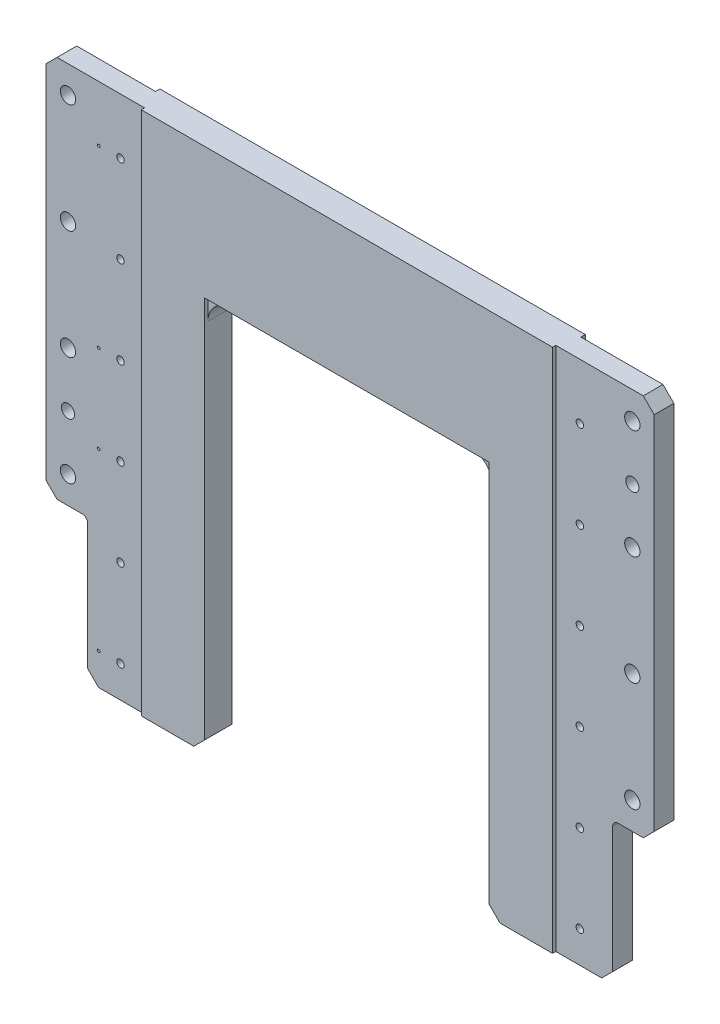
from build123d import *

# Parameters (mm, degrees)
BOSS_EXTRUDE1_DEPTH             = 22
SKETCH2_W                       = 85
SKETCH2_H                       = 480
SKETCH2_W_2                     = 82
CUT_EXTRUDE1_DEPTH              = 4
M8_TAPPED_HOLE1_AT_2_COUNT      = 2
M8_TAPPED_HOLE1_AT_2_PITCH      = 80
M8_TAPPED_HOLE1_AT_3_COUNT      = 2
M8_TAPPED_HOLE1_AT_3_PITCH      = 160
M8_TAPPED_HOLE1_AT_4_COUNT      = 2
M8_TAPPED_HOLE1_AT_4_PITCH      = 240
M8_TAPPED_HOLE1_AT_5_COUNT      = 2
M8_TAPPED_HOLE1_AT_5_PITCH      = 320
M8_TAPPED_HOLE1_AT_6_COUNT      = 2
M8_TAPPED_HOLE1_AT_6_PITCH      = 80
F_14_0_14_DIAMETER_HOLE1_D      = 14
F_7_0_7_DIAMETER_HOLE1_D        = 7
F_7_0_7_DIAMETER_HOLE1_DEPTH    = 4
M3_TAPPED_HOLE1_D               = 2.5
M3_TAPPED_HOLE1_DEPTH           = 18
M3_TAPPED_HOLE1_ON_FACE_2_D     = 2.5
M3_TAPPED_HOLE1_ON_FACE_2_DEPTH = 18
F_12_0_12_DIAMETER_HOLE1_D      = 12
CUT_EXTRUDE2_REACH              = 736.752
SKETCH9_W                       = 38
SKETCH9_H                       = 130
CUT_EXTRUDE2_DIRECTION_2_DEPTH  = 5
FILLET1_R                       = 5
CHAMFER1_SIZE                   = 10
BOSS_EXTRUDE2_DEPTH             = 3


with BuildPart() as part:
    # Sketch1 → Boss-Extrude1 (new body)
    with BuildSketch(Plane.XY):
        with BuildLine():
            Line((0, 10), (0, 470))
            Line((0, 470), (10, 480))
            Line((10, 480), (546, 480))
            Line((546, 480), (556, 470))
            Line((556, 470), (556, 10))
            Line((556, 10), (546, 0))
            Line((546, 0), (418, 0))
            Line((418, 0), (408, 10))
            Line((408, 10), (408, 340))
            ThreePointArc((408, 340), (402.142135624, 354.142135624), (388, 360))
            Line((388, 360), (168, 360))
            ThreePointArc((168, 360), (153.857864376, 354.142135624), (148, 340))
            Line((148, 340), (148, 10))
            Line((148, 10), (138, 0))
            Line((138, 0), (10, 0))
            Line((10, 0), (0, 10))
        make_face()
    extrude(amount=BOSS_EXTRUDE1_DEPTH)

    # Sketch2 → Cut-Extrude1 (cut)
    with BuildSketch(Plane(origin=(0, 0, 0), x_dir=(-1, 0, 0), z_dir=(0, 0, -1))):
        with Locations((-513.5, 240)):
            Rectangle(SKETCH2_W, SKETCH2_H)
        with Locations((-41, 240)):
            Rectangle(SKETCH2_W_2, SKETCH2_H)
    extrude(amount=-CUT_EXTRUDE1_DEPTH, mode=Mode.SUBTRACT)

    # Sketch3 → M8 Tapped Hole1 (revolve, cut)
    with BuildSketch(Plane(origin=(488, 349, 4), x_dir=(0, 1, 0), z_dir=(1, 0, 0))):
        Polygon((0, 0), (0, 21.712990915), (3.4, 19.75), (3.4, 0), align=None)
    m8_tapped_hole1 = revolve(axis=Axis((488, 349, -2.35), (0, 0, 1)), mode=Mode.SUBTRACT)

    # M8 Tapped Hole1 at 2: M8 Tapped Hole1 ×2
    with Locations(*[(0, -i * M8_TAPPED_HOLE1_AT_2_PITCH, 0) for i in range(1, M8_TAPPED_HOLE1_AT_2_COUNT)]):
        add(m8_tapped_hole1, mode=Mode.SUBTRACT)

    # M8 Tapped Hole1 at 3: M8 Tapped Hole1 ×2
    with Locations(*[(0, -i * M8_TAPPED_HOLE1_AT_3_PITCH, 0) for i in range(1, M8_TAPPED_HOLE1_AT_3_COUNT)]):
        add(m8_tapped_hole1, mode=Mode.SUBTRACT)

    # M8 Tapped Hole1 at 4: M8 Tapped Hole1 ×2
    with Locations(*[(0, -i * M8_TAPPED_HOLE1_AT_4_PITCH, 0) for i in range(1, M8_TAPPED_HOLE1_AT_4_COUNT)]):
        add(m8_tapped_hole1, mode=Mode.SUBTRACT)

    # M8 Tapped Hole1 at 5: M8 Tapped Hole1 ×2
    with Locations(*[(0, -i * M8_TAPPED_HOLE1_AT_5_PITCH, 0) for i in range(1, M8_TAPPED_HOLE1_AT_5_COUNT)]):
        add(m8_tapped_hole1, mode=Mode.SUBTRACT)

    # M8 Tapped Hole1 at 6: M8 Tapped Hole1 ×2
    with Locations(*[(0, i * M8_TAPPED_HOLE1_AT_6_PITCH, 0) for i in range(1, M8_TAPPED_HOLE1_AT_6_COUNT)]):
        add(m8_tapped_hole1, mode=Mode.SUBTRACT)

    # Mirror1: M8 Tapped Hole1 across plane
    add(m8_tapped_hole1.mirror(Plane(origin=(278, 0, 0), x_dir=(0, 0, 1), z_dir=(1, 0, 0))), mode=Mode.SUBTRACT)

    # Mirror1 copy 1 sketch → Mirror1 copy 1 (revolve, cut)
    with BuildSketch(Plane(origin=(68, 269, 4), x_dir=(0, 1, 0), z_dir=(-1, 0, 0))):
        Polygon((0, 0), (0, -21.712990915), (3.4, -19.75), (3.4, 0), align=None)
    revolve(axis=Axis((68, 269, -2.35), (0, 0, -1)), mode=Mode.SUBTRACT)

    # Mirror1 copy 2 sketch → Mirror1 copy 2 (revolve, cut)
    with BuildSketch(Plane(origin=(68, 189, 4), x_dir=(0, 1, 0), z_dir=(-1, 0, 0))):
        Polygon((0, 0), (0, -21.712990915), (3.4, -19.75), (3.4, 0), align=None)
    revolve(axis=Axis((68, 189, -2.35), (0, 0, -1)), mode=Mode.SUBTRACT)

    # Mirror1 copy 3 sketch → Mirror1 copy 3 (revolve, cut)
    with BuildSketch(Plane(origin=(68, 109, 4), x_dir=(0, 1, 0), z_dir=(-1, 0, 0))):
        Polygon((0, 0), (0, -21.712990915), (3.4, -19.75), (3.4, 0), align=None)
    revolve(axis=Axis((68, 109, -2.35), (0, 0, -1)), mode=Mode.SUBTRACT)

    # Mirror1 copy 4 sketch → Mirror1 copy 4 (revolve, cut)
    with BuildSketch(Plane(origin=(68, 29, 4), x_dir=(0, 1, 0), z_dir=(-1, 0, 0))):
        Polygon((0, 0), (0, -21.712990915), (3.4, -19.75), (3.4, 0), align=None)
    revolve(axis=Axis((68, 29, -2.35), (0, 0, -1)), mode=Mode.SUBTRACT)

    # Mirror1 copy 5 sketch → Mirror1 copy 5 (revolve, cut)
    with BuildSketch(Plane(origin=(68, 429, 4), x_dir=(0, 1, 0), z_dir=(-1, 0, 0))):
        Polygon((0, 0), (0, -21.712990915), (3.4, -19.75), (3.4, 0), align=None)
    revolve(axis=Axis((68, 429, -2.35), (0, 0, -1)), mode=Mode.SUBTRACT)

    # Ø14.0 (14) Diameter Hole1 (through all)
    with Locations(Plane(origin=(536, 455, 4), x_dir=(-1, 0, 0), z_dir=(0, 0, -1))):
        with Locations((0, 0), (0, -100), (0, -200), (0, -300)):
            f_14_0_14_diameter_hole1 = Hole(F_14_0_14_DIAMETER_HOLE1_D / 2)

    # Mirror2: Ø14.0 (14) Diameter Hole1 across plane
    add(f_14_0_14_diameter_hole1.mirror(Plane.ZY.offset(-278)), mode=Mode.SUBTRACT)

    # Ø7.0 (7) Diameter Hole1
    with Locations(Plane(origin=(48, 429, 4), x_dir=(-1, 0, 0), z_dir=(0, 0, -1))):
        with Locations((0, 0), (0, -160), (0, -240), (0, -400)):
            Hole(F_7_0_7_DIAMETER_HOLE1_D / 2, depth=F_7_0_7_DIAMETER_HOLE1_DEPTH)

    # M3 Tapped Hole1
    with Locations(Plane(origin=(48, 429, 4), x_dir=(-1, 0, 0), z_dir=(0, 0, -1))):
        with Locations((0, 0), (0, -240)):
            Hole(M3_TAPPED_HOLE1_D / 2, depth=M3_TAPPED_HOLE1_DEPTH)

    # M3 Tapped Hole1 on face 2
    with Locations(Plane(origin=(48, 269, 8), x_dir=(-1, 0, 0), z_dir=(0, 0, -1))):
        with Locations((0, 0), (0, -240)):
            Hole(M3_TAPPED_HOLE1_ON_FACE_2_D / 2, depth=M3_TAPPED_HOLE1_ON_FACE_2_DEPTH)

    # Ø12.0 (12) Diameter Hole1 (through all)
    with Locations(Plane(origin=(20, 205, 4), x_dir=(-1, 0, 0), z_dir=(0, 0, -1))):
        with Locations((0, 0), (-516, 200)):
            Hole(F_12_0_12_DIAMETER_HOLE1_D / 2)

    # Sketch9 → Cut-Extrude2 (cut, up to next)
    with BuildSketch(Plane(origin=(0, 0, 4), x_dir=(-1, 0, 0), z_dir=(0, 0, -1)), mode=Mode.PRIVATE) as cut_extrude2_sk1:
        with Locations((-537, 65)):
            Rectangle(SKETCH9_W, SKETCH9_H)
    cut_extrude2_tool1 = extrude(cut_extrude2_sk1.sketch, amount=-CUT_EXTRUDE2_REACH, mode=Mode.PRIVATE) & part.part
    # Sketch9 → Cut-Extrude2 (cut, up to next)
    with BuildSketch(Plane(origin=(0, 0, 4), x_dir=(-1, 0, 0), z_dir=(0, 0, -1)), mode=Mode.PRIVATE) as cut_extrude2_sk2:
        with Locations((-19, 65)):
            Rectangle(SKETCH9_W, SKETCH9_H)
    cut_extrude2_tool2 = extrude(cut_extrude2_sk2.sketch, amount=-CUT_EXTRUDE2_REACH, mode=Mode.PRIVATE) & part.part
    add(cut_extrude2_tool1.solids().sort_by_distance((537, 65, 4))[0], mode=Mode.SUBTRACT)
    add(cut_extrude2_tool2.solids().sort_by_distance((19, 65, 4))[0], mode=Mode.SUBTRACT)

    # Sketch9 → Cut-Extrude2 direction 2 (cut)
    with BuildSketch(Plane(origin=(0, 0, 4), x_dir=(-1, 0, 0), z_dir=(0, 0, -1))):
        with Locations((-537, 65)):
            Rectangle(SKETCH9_W, SKETCH9_H)
        with Locations((-19, 65)):
            Rectangle(SKETCH9_W, SKETCH9_H)
    extrude(amount=CUT_EXTRUDE2_DIRECTION_2_DEPTH, mode=Mode.SUBTRACT)

    # Fillet1
    fillet1_edges = [part.edges().sort_by_distance(p)[0] for p in [
        (518, 130, 13),
        (38, 130, 13),
    ]]
    fillet(fillet1_edges, radius=FILLET1_R)

    # Chamfer1
    chamfer1_edges = [part.edges().sort_by_distance(p)[0] for p in [
        (556, 130, 13),
        (518, 0, 13),
        (38, 0, 13),
        (0, 130, 13),
    ]]
    chamfer(chamfer1_edges, length=CHAMFER1_SIZE)

    # Sketch10 → Boss-Extrude2 (add)
    with BuildSketch(Plane.XY.offset(22)):
        Polygon((90, 480), (90, 0), (138, 0), (148, 10), (148, 360), (408, 360), (408, 10), (418, 0), (466, 0), (466, 480), align=None)
    extrude(amount=BOSS_EXTRUDE2_DEPTH)


solid = part.part
